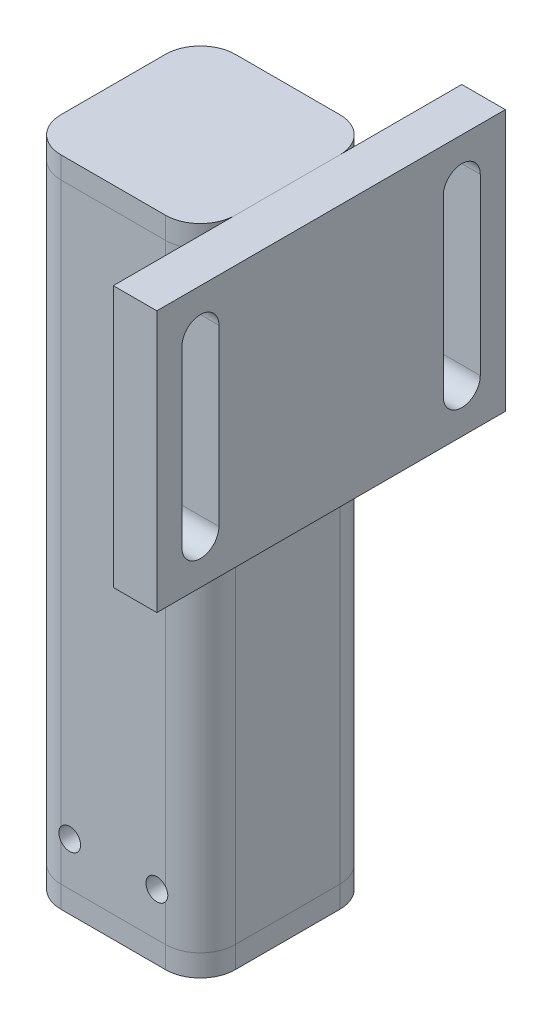
SolidWorks part; units mm, degrees
ref_plane "前视基准面" through (0, 0, 0) normal (0, 0, 1) x (1, 0, 0)
ref_plane "上视基准面" through (0, 0, 0) normal (0, 1, 0) x (1, 0, 0)
ref_plane "右视基准面" through (0, 0, 0) normal (1, 0, 0) x (0, 0, -1)
sketch "草图1" plane through (0, 0, 0) normal (1, 0, 0) x (0, 0, -1)
  line L0 (0, 0) -> (0, 150)
  dimension "D1" = 150
other "方管 40 X 40 X 4.0(1)"
ref_plane "基准面1" through (0, 0, 0) normal (0, 1, 0) x (0, 0, 1)
sketch "Sketch1" plane through (0, 0, 0) normal (0, 1, 0) x (0, 0, 1)
  line L0 (-12, -16) -> (12, -16)
  line L1 (-16, -12) -> (-16, 12)
  line L2 (12, 16) -> (-12, 16)
  line L3 (16, 12) -> (16, -12)
  line L4 (-12, -20) -> (12, -20)
  line L5 (-20, -12) -> (-20, 12)
  line L6 (12, 20) -> (-12, 20)
  line L7 (20, 12) -> (20, -12)
  line L8 (-20, 0) -> (-16, 0) construction
  line L9 (-16, 0) -> (16, 0) construction
  line L10 (16, 0) -> (20, 0) construction
  line L12 (0, 20) -> (0, 16) construction
  line L13 (0, 16) -> (0, -16) construction
  line L14 (0, -16) -> (0, -20) construction
  arc A0 (20, 12) -> (12, 20) centre (12, 12) ccw
  arc A1 (12, -20) -> (20, -12) centre (12, -12) ccw
  arc A2 (-20, -12) -> (-12, -20) centre (-12, -12) ccw
  arc A3 (-12, 20) -> (-20, 12) centre (-12, 12) ccw
  arc A4 (-12, 16) -> (-16, 12) centre (-12, 12) ccw
  arc A5 (16, 12) -> (12, 16) centre (12, 12) ccw
  arc A6 (12, -16) -> (16, -12) centre (12, -12) ccw
  arc A7 (-16, -12) -> (-12, -16) centre (-12, -12) ccw
  point P2 (-20, 20)
  point P33 (-20, -20)
  point P34 (20, -20)
  point P36 (20, 20)
  point P37 (0, 0)
  dimension "D1" = 8
  dimension "Thickness" = 4
  dimension "V_leg" = 40
  dimension "H_leg" = 40
sketch "草图3" plane through (20, 0, 0) normal (1, 0, 0) x (0, 0, -1)
  line L0 (0, 0) -> (0, 150) construction
  line L1 (-40, 150) -> (40, 150)
  line L2 (-40, 150) -> (-40, 90)
  line L3 (-40, 90) -> (40, 90)
  line L4 (40, 150) -> (40, 90)
  line L5 (-40, 150) -> (40, 90) construction
  line L6 (-40, 90) -> (40, 150) construction
  line L7 (-12, 150) -> (12, 150) construction
  point P0 (0, 120)
  dimension "D1" = 60
  dimension "D2" = 80
extrude "凸台-拉伸1" add sketch "草图3" along normal blind 10 separate body
sketch "草图12" plane through (30, 0, 0) normal (1, 0, 0) x (0, 0, -1)
  line L0 (-30, 140) -> (-30, 100) construction
  line L1 (-25.75, 140) -> (-25.75, 100)
  line L2 (-34.25, 140) -> (-34.25, 100)
  line L3 (30, 140) -> (30, 100) construction
  line L4 (34.25, 140) -> (34.25, 100)
  line L5 (25.75, 140) -> (25.75, 100)
  line L6 (0, 150) -> (0, 222.0658) construction
  line L7 (0, 0) -> (0, 150) construction
  line L8 (-40, 120) -> (68.4695, 120) construction
  line L9 (-40, 150) -> (-40, 90) construction
  arc A0 (-25.75, 140) -> (-34.25, 140) centre (-30, 140) ccw
  arc A1 (-34.25, 100) -> (-25.75, 100) centre (-30, 100) ccw
  arc A2 (34.25, 140) -> (25.75, 140) centre (30, 140) ccw
  arc A3 (25.75, 100) -> (34.25, 100) centre (30, 100) ccw
  point P2 (-30, 120)
  point P7 (30, 120)
  dimension "D1" = 40
  dimension "D2" = 8.5
  dimension "D3" = 60
extrude "切除-拉伸2" cut sketch "草图12" against normal through all
hole_wizard "M6 螺纹孔1" positions "草图13" profile "草图14" tap size "M6" standard "GB" end condition through all
sketch "草图13" plane through (0, 0, 20) normal (0, 0, 1) x (1, 0, 0)
  line L1 (0, 0) -> (0, 29.0944) construction
  line L2 (0, 0) -> (0, 150) construction
  line L4 (-12, 0) -> (12, 0) construction
  point P0 (-10, 15)
  point P2 (10, 15)
  dimension "D1" = 20
  dimension "D2" = 15
sketch "草图14" plane through (-10, 15, 20) normal (1, 0, 0) x (0, -1, 0)
  line L0 (0, 0) -> (0, 60)
  line L1 (0, 60) -> (2.5, 60)
  line L2 (2.5, 60) -> (2.5, 0)
  line L5 (2.5, 0) -> (0, 0)
  line L11 (0, -6.35) -> (0, 107.95) construction
  dimension "通孔螺纹孔钻头直径" = 5
  dimension "通孔螺纹孔钻头深度" = 60
cosmetic thread "孔螺蚊线6" parameters "D2"=6
cosmetic thread "孔螺蚊线7" parameters "D2"=6
other "顶端盖1" parameters "D1"=5, "D2"=3, "D3"=8
hole_wizard "M6 螺纹孔2" positions "草图16" profile "草图17" tap size "M6" standard "GB"
sketch "草图16" plane through (0, 0, 0) normal (0, -1, 0) x (-1, 0, 0)
  line L0 (0, 0) -> (0, 10.5465) construction
  point P0 (10, 0)
  point P2 (-10, 0)
  dimension "D1" = 20
sketch "草图17" plane through (-10, 0, 0) normal (1, 0, 0) x (0, 0, -1)
  line L0 (0, 0) -> (0, 16.5022)
  line L1 (0, 16.5022) -> (2.5, 15)
  line L2 (2.5, 15) -> (2.5, 0)
  line L5 (2.5, 0) -> (0, 0)
  line L10 (0, 16.5022) -> (-2.5, 15) construction
  line L11 (0, -6.35) -> (0, 107.95) construction
  dimension "螺纹孔钻头直径" = 5
  dimension "螺纹孔钻头深度" = 15
  dimension "导头角度" = 118
cosmetic thread "孔螺蚊线8" parameters "D1"=5, "D2"=6
cosmetic thread "孔螺蚊线9" parameters "D1"=5, "D2"=6
other "顶端盖2" parameters "D1"=5, "D2"=3, "D3"=8
